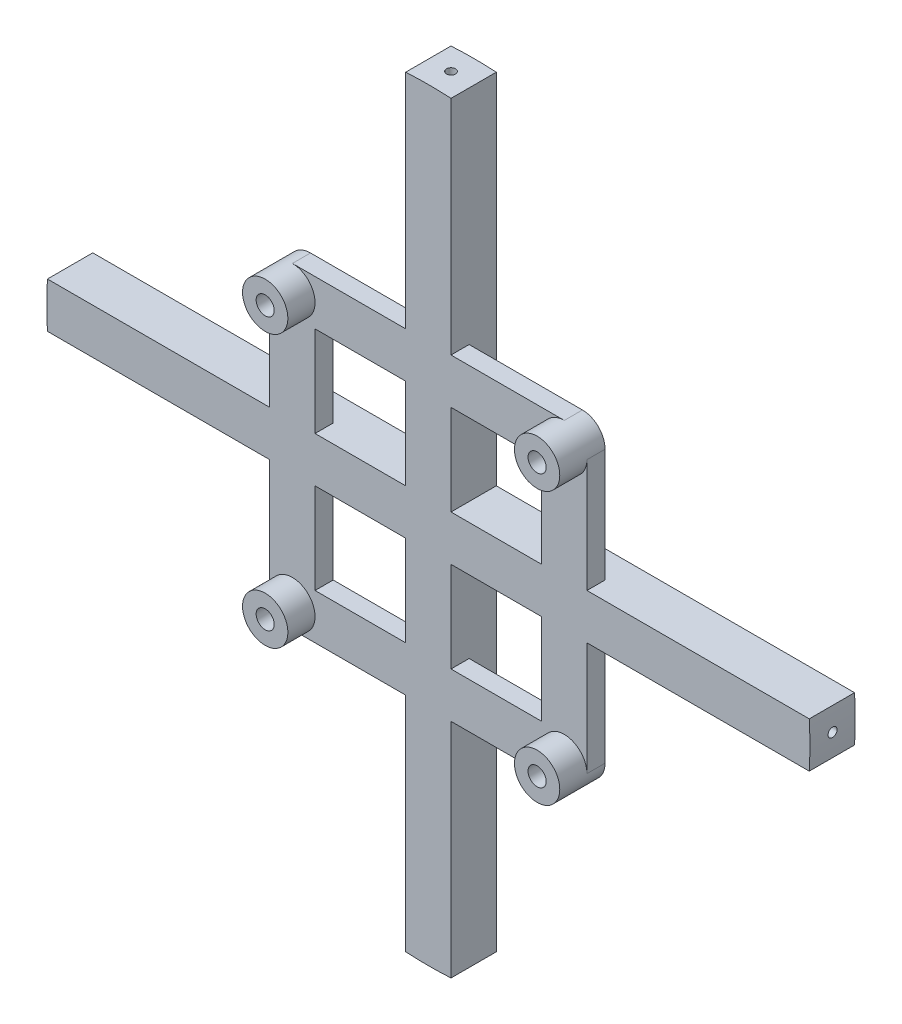
SolidWorks part; units mm, degrees
ref_plane "Front Plane" through (0, 0, 0) normal (0, 0, 1) x (1, 0, 0)
ref_plane "Top Plane" through (0, 0, 0) normal (0, 1, 0) x (1, 0, 0)
ref_plane "Right Plane" through (0, 0, 0) normal (1, 0, 0) x (0, 0, -1)
other "Configuration Table"
sketch "Sketch1" plane through (0, 0, 0) normal (0, 0, 1) x (1, 0, 0)
  line L0 (-50.8683, 0) -> (53.6152, 0) construction
  line L1 (0, 46.8715) -> (0, -47.4063) construction
  line L2 (-42.0257, 2.5) -> (-2.5, 2.5)
  line L3 (-2.5, 2.5) -> (-2.5, 42.0257)
  line L4 (2.5, 42.0257) -> (2.5, 2.5)
  line L5 (2.5, 2.5) -> (42.0257, 2.5)
  line L6 (42.0257, -2.5) -> (2.5, -2.5)
  line L7 (2.5, -2.5) -> (2.5, -42.0257)
  line L8 (-42.0257, -2.5) -> (-2.5, -2.5)
  line L9 (-2.5, -2.5) -> (-2.5, -42.0257)
  arc A0 (-42.0257, 2.5) -> (-42.0257, -2.5) centre (0, 0) ccw
  arc A1 (2.5, 42.0257) -> (-2.5, 42.0257) centre (0, 0) ccw
  arc A2 (42.0257, -2.5) -> (42.0257, 2.5) centre (0, 0) ccw
  arc A3 (-2.5, -42.0257) -> (2.5, -42.0257) centre (0, 0) ccw
  dimension "D1" = 84.2
  dimension "D2" = 5
  dimension "D3" = 2.5
  dimension "D4" = 5
  dimension "D5" = 2.5
  dimension "D6" = 5
  dimension "D7" = 2.5
  dimension "D8" = 2.5
extrude "Boss-Extrude1" add sketch "Sketch1" along normal blind 5
sketch "Sketch2" plane through (0, 0, 5) normal (0, 0, 1) x (1, 0, 0)
  line L0 (2.5, 12.5) -> (12.5, 12.5)
  line L1 (-12.5, 12.5) -> (-2.5, 12.5)
  line L2 (-12.5, 12.5) -> (-12.5, 2.5)
  line L3 (-12.5, -12.5) -> (-2.5, -12.5)
  line L4 (12.5, 12.5) -> (12.5, 2.5)
  line L5 (-17.5, 17.5) -> (-2.5, 17.5)
  line L6 (-17.5, 17.5) -> (-17.5, 2.5)
  line L7 (-17.5, -17.5) -> (-2.5, -17.5)
  line L8 (17.5, 17.5) -> (17.5, 2.5)
  line L9 (2.5, 17.5) -> (17.5, 17.5)
  line L10 (0, 0) -> (52.6329, 0) construction
  line L11 (0, 0) -> (0, -46.6261) construction
  line L12 (-12.5, -2.5) -> (-12.5, -12.5)
  line L13 (12.5, -2.5) -> (12.5, -12.5)
  line L14 (-17.5, -2.5) -> (-17.5, -17.5)
  line L15 (17.5, -2.5) -> (17.5, -17.5)
  line L16 (2.5, -12.5) -> (12.5, -12.5)
  line L17 (2.5, -17.5) -> (17.5, -17.5)
  line L20 (-2.5, 42.0257) -> (-2.5, 2.5)
  line L21 (-2.5, 2.5) -> (-42.0257, 2.5)
  line L22 (-42.0257, -2.5) -> (-2.5, -2.5)
  line L23 (-2.5, -2.5) -> (-2.5, -42.0257)
  line L24 (2.5, -42.0257) -> (2.5, -2.5)
  line L25 (2.5, -2.5) -> (42.0257, -2.5)
  line L26 (42.0257, 2.5) -> (2.5, 2.5)
  line L27 (2.5, 2.5) -> (2.5, 42.0257)
  line L28 (-2.5, 17.5) -> (-2.5, 12.5)
  line L29 (-12.5, 2.5) -> (-17.5, 2.5)
  line L30 (-17.5, -2.5) -> (-12.5, -2.5)
  line L31 (-2.5, -12.5) -> (-2.5, -17.5)
  line L32 (2.5, -17.5) -> (2.5, -12.5)
  line L33 (12.5, -2.5) -> (17.5, -2.5)
  line L34 (17.5, 2.5) -> (12.5, 2.5)
  line L35 (2.5, 12.5) -> (2.5, 17.5)
  arc A4 (2.5, 42.0257) -> (-2.5, 42.0257) centre (0, 0) ccw
  arc A5 (-42.0257, 2.5) -> (-42.0257, -2.5) centre (0, 0) ccw
  arc A6 (-2.5, -42.0257) -> (2.5, -42.0257) centre (0, 0) ccw
  arc A7 (42.0257, -2.5) -> (42.0257, 2.5) centre (0, 0) ccw
  dimension "D1" = 25
  dimension "D2" = 35
  dimension "D3" = 0
extrude "Boss-Extrude2" add sketch "Sketch2" against normal blind 2 separate body
sketch "Sketch3" plane through (0, 0, 5) normal (0, 0, 1) x (1, 0, 0)
  line L0 (17.5, 17.5) -> (2.5, 17.5) construction
  line L1 (17.5, 2.5) -> (17.5, 17.5) construction
  line L2 (0, 0) -> (32.3054, 0) construction
  line L3 (0, 0) -> (0, 19.4474) construction
  circle A0 centre (15, 15) radius 2.5
  circle A1 centre (15, 15) radius 1
  dimension "D1" = 5
  dimension "D2" = 2
  dimension "D3" = 2.5
  dimension "D4" = 2.5
extrude "Cut-Extrude1" cut sketch "Sketch3" against normal through all contours A1
sketch "Sketch5" plane through (0, 0, 5) normal (0, 0, 1) x (1, 0, 0)
  circle A0 centre (15, 15) radius 1 construction
  circle A1 centre (15, 15) radius 2.5 construction
  circle A2 centre (15, 15) radius 1
  circle A3 centre (15, 15) radius 2.5
extrude "Boss-Extrude3" add sketch "Sketch5" along normal blind 3
sketch "Sketch6" plane through (0, 0, 5) normal (0, 0, 1) x (1, 0, 0)
  line L0 (17.5, 15) -> (17.5, 17.5) construction
  line L1 (17.5, 17.5) -> (15, 17.5) construction
  line L2 (17.5, 15) -> (17.5, 17.5)
  line L3 (17.5, 17.5) -> (15, 17.5)
  line L11 (2.5, 17.5) -> (2.5, 42.0257)
  line L12 (-2.5, 42.0257) -> (-2.5, 2.5)
  line L13 (-2.5, 2.5) -> (-42.0257, 2.5)
  line L14 (-42.0257, -2.5) -> (-2.5, -2.5)
  line L15 (-2.5, -2.5) -> (-2.5, -42.0257)
  line L16 (2.5, -42.0257) -> (2.5, -2.5)
  line L17 (2.5, -2.5) -> (42.0257, -2.5)
  line L18 (42.0257, 2.5) -> (17.5, 2.5)
  line L21 (2.5, 17.5) -> (2.5, 42.0257)
  line L22 (-2.5, 42.0257) -> (-2.5, 2.5)
  line L23 (-2.5, 2.5) -> (-42.0257, 2.5)
  line L24 (-42.0257, -2.5) -> (-2.5, -2.5)
  line L25 (-2.5, -2.5) -> (-2.5, -42.0257)
  line L26 (2.5, -42.0257) -> (2.5, -2.5)
  line L27 (2.5, -2.5) -> (42.0257, -2.5)
  line L28 (42.0257, 2.5) -> (17.5, 2.5)
  line L34 (15, 17.5) -> (2.5, 17.5)
  line L35 (15, 17.5) -> (2.5, 17.5)
  line L36 (17.5, 2.5) -> (17.5, 15)
  line L37 (17.5, 2.5) -> (17.5, 15)
  circle A0 centre (15, 15) radius 2.5 construction
  arc A1 (17.5, 15) -> (15, 17.5) centre (15, 15) ccw
  arc A6 (2.5, 42.0257) -> (-2.5, 42.0257) centre (0, 0) ccw
  arc A7 (-42.0257, 2.5) -> (-42.0257, -2.5) centre (0, 0) ccw
  arc A8 (-2.5, -42.0257) -> (2.5, -42.0257) centre (0, 0) ccw
  arc A9 (42.0257, -2.5) -> (42.0257, 2.5) centre (0, 0) ccw
  arc A11 (2.5, 42.0257) -> (-2.5, 42.0257) centre (0, 0) ccw
  arc A12 (-42.0257, 2.5) -> (-42.0257, -2.5) centre (0, 0) ccw
  arc A13 (-2.5, -42.0257) -> (2.5, -42.0257) centre (0, 0) ccw
  arc A14 (42.0257, -2.5) -> (42.0257, 2.5) centre (0, 0) ccw
  arc A17 (15, 17.5) -> (17.5, 15) centre (15, 15) ccw
  dimension "D1" = 0
extrude "Cut-Extrude2" cut sketch "Sketch6" against normal through all contours A1 L2 L3
sketch "Sketch12" plane through (0, 0, 5) normal (0, 0, 1) x (1, 0, 0)
  line L0 (17.5, -17.5) -> (17.5, -2.5) construction
  line L1 (2.5, -17.5) -> (17.5, -17.5) construction
  line L2 (0, 0) -> (40.7178, 0) construction
  line L3 (0, 0) -> (0, -22.0912) construction
  circle A1 centre (15, -15) radius 2.5
  circle A2 centre (-15, -15) radius 2.5
  circle A3 centre (-15, 15) radius 2.5
  dimension "D1" = 5
  dimension "D3" = 2.5
  dimension "D4" = 2.5
extrude "Boss-Extrude4" add sketch "Sketch12" along normal blind 3
sketch "Sketch13" plane through (0, 0, 8) normal (0, 0, 1) x (1, 0, 0)
  line L0 (0, 0) -> (30.3471, 0) construction
  line L1 (0, 0) -> (0, -18.5964) construction
  circle A0 centre (15, -15) radius 1
  circle A1 centre (-15, -15) radius 1
  circle A2 centre (-15, 15) radius 1
  dimension "D1" = 2
extrude "Cut-Extrude3" cut sketch "Sketch13" against normal through all
sketch "Sketch14" plane through (0, 0, 5) normal (0, 0, 1) x (1, 0, 0)
  line L0 (-15, 17.5) -> (-17.5, 17.5) construction
  line L1 (-17.5, 17.5) -> (-17.5, 15) construction
  line L2 (-17.5, -15) -> (-17.5, -17.5) construction
  line L3 (-17.5, -17.5) -> (-15, -17.5) construction
  line L4 (15, -17.5) -> (17.5, -17.5) construction
  line L5 (17.5, -17.5) -> (17.5, -15) construction
  line L6 (-15, 17.5) -> (-17.5, 17.5)
  line L7 (-17.5, 17.5) -> (-17.5, 15)
  line L8 (-17.5, -15) -> (-17.5, -17.5)
  line L9 (-17.5, -17.5) -> (-15, -17.5)
  line L10 (15, -17.5) -> (17.5, -17.5)
  line L11 (17.5, -17.5) -> (17.5, -15)
  arc A0 (-15, 17.5) -> (-17.5, 15) centre (-15, 15) ccw construction
  arc A1 (-17.5, -15) -> (-15, -17.5) centre (-15, -15) ccw construction
  arc A2 (15, -17.5) -> (17.5, -15) centre (15, -15) ccw construction
  arc A3 (-15, 17.5) -> (-17.5, 15) centre (-15, 15) ccw
  arc A4 (-17.5, -15) -> (-15, -17.5) centre (-15, -15) ccw
  arc A5 (15, -17.5) -> (17.5, -15) centre (15, -15) ccw
extrude "Cut-Extrude4" cut sketch "Sketch14" against normal through all
sketch "Sketch17" plane through (0, 0, 0) normal (0, 1, 0) x (1, 0, 0)
  line L0 (0, -4.4) -> (0, 4.4) construction
  line L2 (2.5, 0) -> (-2.5, 0) construction
  circle A0 centre (0, -2.5) radius 0.5
  dimension "D1" = 1
  dimension "D2" = 2.5
extrude "Cut-Extrude5" cut sketch "Sketch17" against normal through all and the other way through all
sketch "Sketch18" plane through (0, 0, 0) normal (1, 0, 0) x (0, 0, -1)
  line L0 (4.4, 0) -> (-4.4, 0) construction
  line L1 (0, -2.5) -> (0, 2.5) construction
  circle A0 centre (-2.5, 0) radius 0.5
  dimension "D1" = 1
  dimension "D2" = 2.5
extrude "Cut-Extrude6" cut sketch "Sketch18" against normal through all and the other way through all
